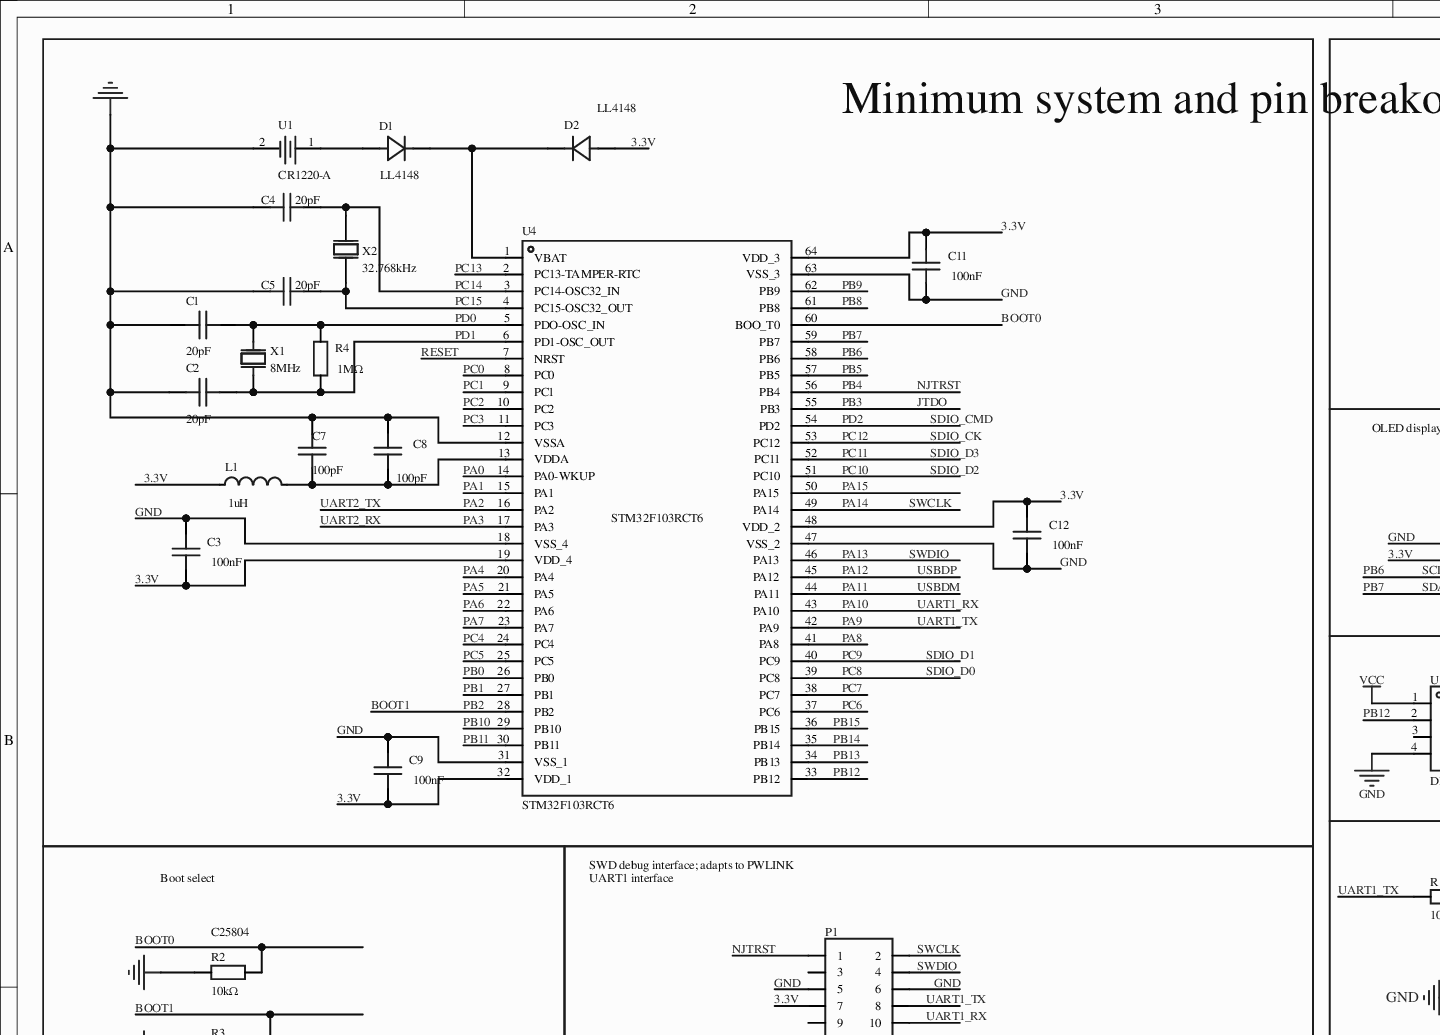
[diagram p0: MISC52064-3.schdoc, top left]
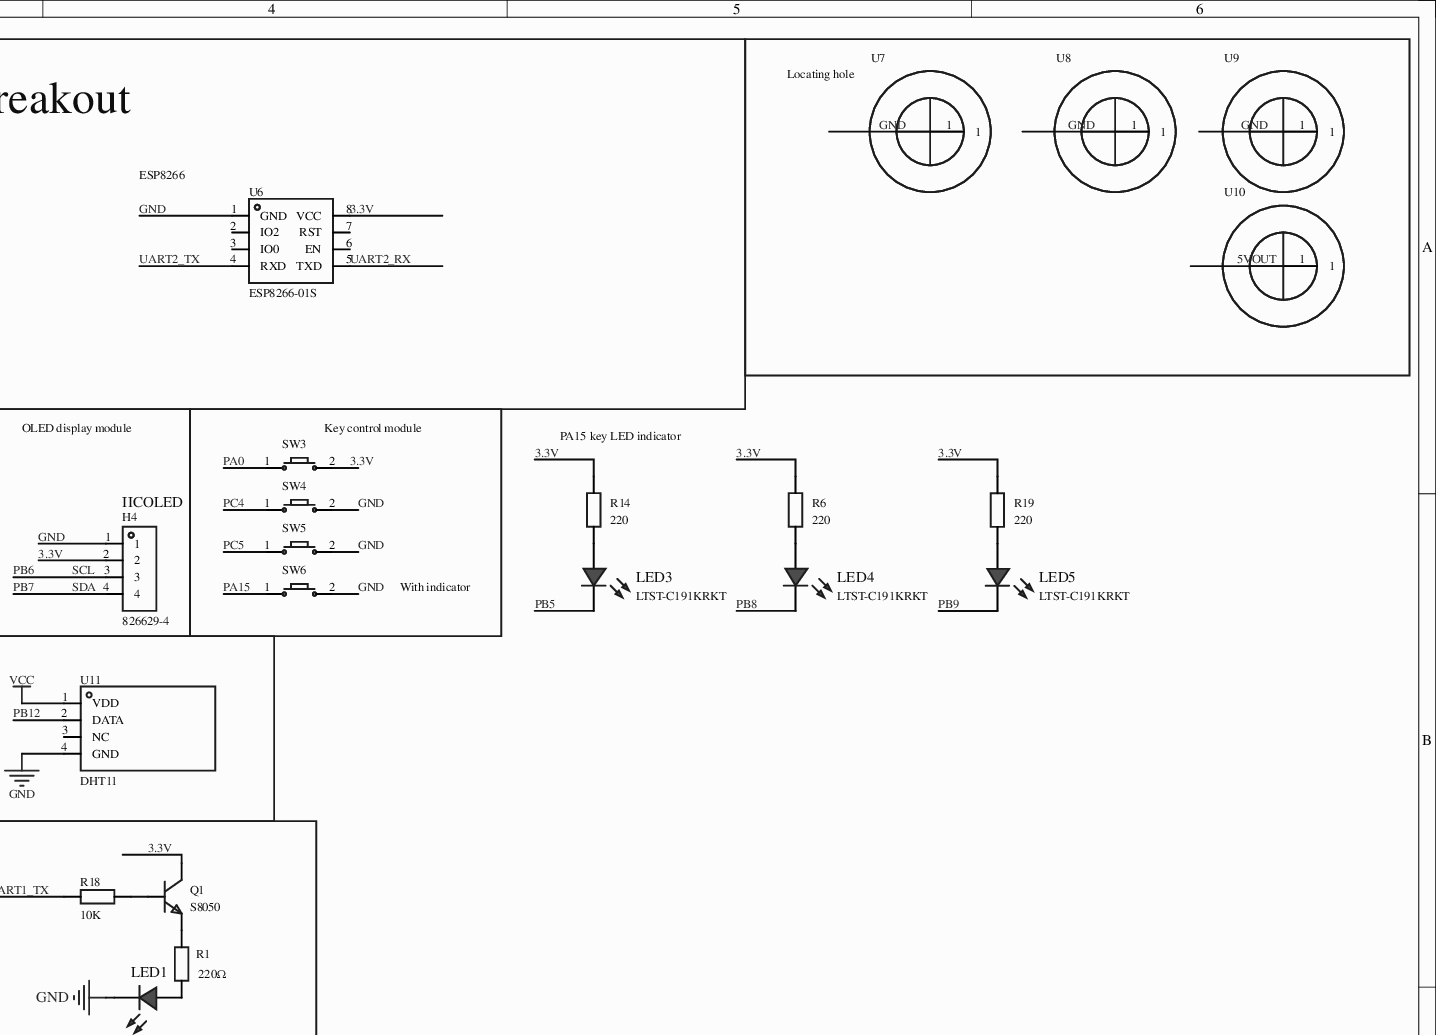
[diagram p1: MISC52064-3.schdoc, top right]
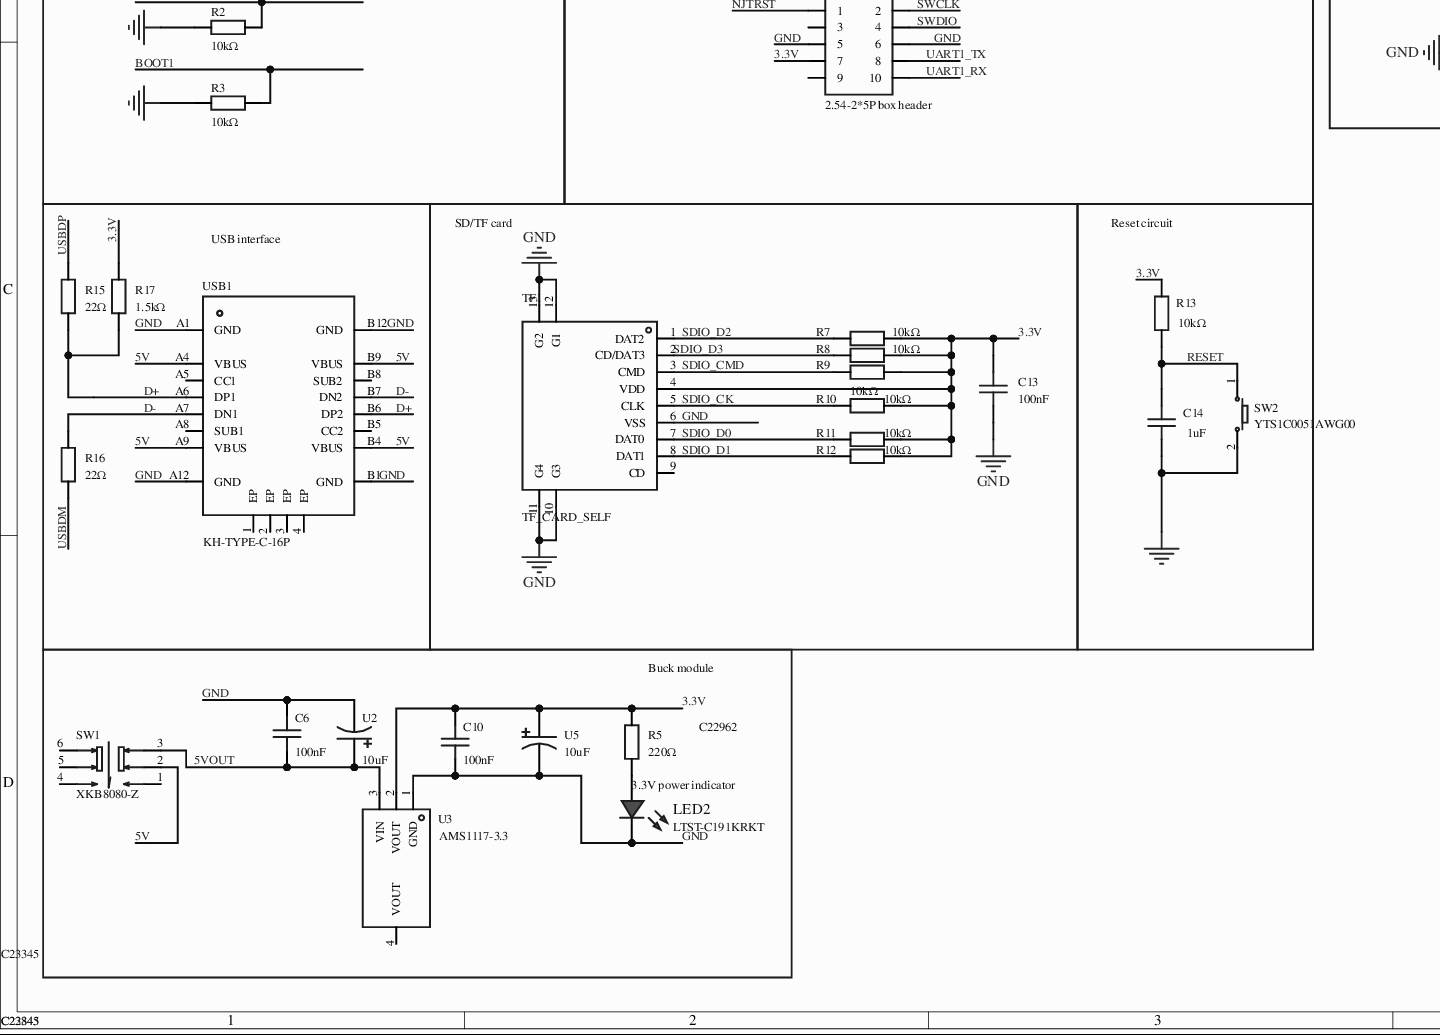
[diagram p2: MISC52064-3.schdoc, bottom left]
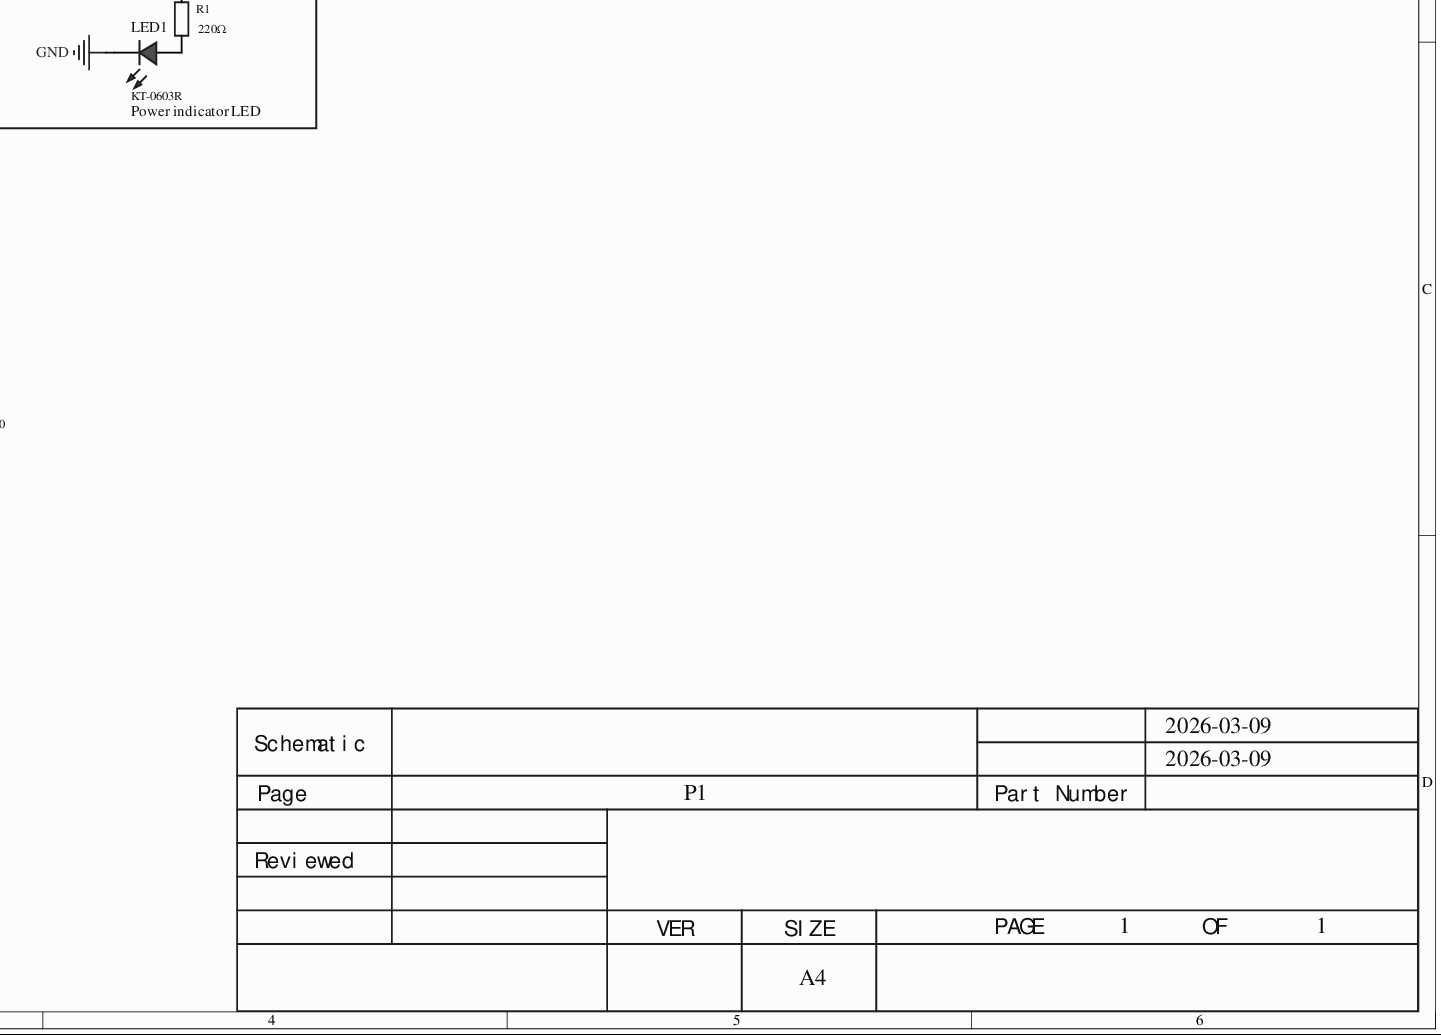
[diagram p3: MISC52064-3.schdoc, bottom right]
# Altium project MISC52064-2.PrjPcb
1 sheet, 65 parts. Net scope: global (net labels, ports and power ports of the same name join across sheets).
Board file: MISC52064.pcbdoc

## Sheet MISC52064-3.schdoc
size 420 x 298 mm; Version: V1.0; @Project Name: MISC52064; @Page Count: 1; @Update Date: 2026-03-09; @Create Date: 2026-03-09; @Schematic Name: MISC52064; @Page No: 1; @Board Name: MISC52064; @Create Time: 16:36:21; @Update Time: 22:44:30

### Parts
C1  20pF  [C0603]
C2  20pF  [C0603]
C3  100nF  [C0603]
C4  20pF  [C0603]
C5  20pF  [C0603]
C6  100nF  [C0603]
C7  100pF  [C0603]
C8  100pF  [C0603]
C9  100nF  [C0603]
C10  100nF  [C0603]
C11  100nF  [C0603]
C12  100nF  [C0603]
C13  100nF  [C0603]
C14  1uF  [C0603]
D1  LL4148  [LL-34_L3.5-W1.5-RD]
D2  LL4148  [LL-34_L3.5-W1.5-RD]
H4  826629-4  用途: IICOLED  [HDR-TH_4P-P2.54-V-M-1]
L1  1uH  [L0603]
LED1  KT-0603R  用途: Power indicator LED  [LED0603-RD]
LED2  LTST-C191KRKT  [LED0603-RD]
LED3  LTST-C191KRKT  [LED0603-RD]
LED4  LTST-C191KRKT  [LED0603-RD]
LED5  LTST-C191KRKT  [LED0603-RD]
P1  2.54-2*5P box header  [IDC-TH_10P-P2.54_C5665]
Q1  S8050  [SOT-23-3_L2.9-W1.3-P1.90-LS2.4-BR]
R1  220Ω  [R0603]
R2  10kΩ  Supplier Part: C25804  [R0603]
R3  10kΩ  [R0603]
R4  1MΩ  [R0603]
R5  220Ω  Supplier Part: C22962  [R0603]
R6  220  [R0603]
R7  10kΩ  [R0603]
R8  10kΩ  [R0603]
R9  10kΩ  [R0603]
R10  10kΩ  [R0603]
R11  10kΩ  [R0603]
R12  10kΩ  [R0603]
R13  10kΩ  [R0603]
R14  220  [R0603]
R15  22Ω  Supplier Part: C23345  [R0603]
R16  22Ω  Supplier Part: C23345  [R0603]
R17  1.5kΩ  Supplier Part: C22843  [R0603]
R18  10K  [R0603]
R19  220  [R0603]
SW1  XKB8080-Z  [SW-TH_6P-L8.0-W8.0-P2.50]
SW2  YTS1C0051AWG00  [SW-SMD_L6.1-W3.6-LS8.0]
SW3  YTS1C0051AWG00  [SW-SMD_L6.1-W3.6-LS8.0]  (value not drawn)
SW4  YTS1C0051AWG00  [SW-SMD_L6.1-W3.6-LS8.0]  (value not drawn)
SW5  YTS1C0051AWG00  [SW-SMD_L6.1-W3.6-LS8.0]  (value not drawn)
SW6  YTS1C0051AWG00  [SW-SMD_L6.1-W3.6-LS8.0]  (value not drawn)
TF1  TF_CARD_SELF  [TF-SMD_TF-15-15]
U1  CR1220-A  [BAT-SMD_CR1220-2]
U2  10uF  [CASE-A_3216]
U3  AMS1117-3.3  [SOT-223-3_L6.5-W3.4-P2.30-LS7.0-BR]
U4  STM32F103RCT6  [LQFP-64_L10.0-W10.0-P0.50-LS12.0-BL]
U5  10uF  [CASE-A_3216]
U6  ESP8266-01S  [WIFIM-TH_ESP8266-01S]
U7  (no value)  [M3_花孔]
U8  (no value)  [M3_花孔]
U9  (no value)  [M3_花孔]
U10  (no value)  [M3_花孔]
U11  DHT11  [SENSOR-TH_DHT11]
USB1  KH-TYPE-C-16P  [USB-C-SMD_KH-TYPE-C-16P]
X1  8MHz  [HC-49S_L11.4-W4.8]
X2  32.768kHz  [OSC-TH_BD2.0-P0.70-D0.3]

### Blocks framed on the sheet
Minimum system and pin breakout: C1-C5 C7-C9 C11 C12 D1 D2 L1 R4 U1 U4 X1 X2
ESP8266: U6
Locating hole: U7-U10
OLED display module: H4
Boot select: R2 R3
USB interface: R15-R17 USB1
SD/TF card: C13 R7-R12 TF1
Reset circuit: C14 R13 SW2

### Nets
GND: C1.1 C2.1 C3.2 C4.1 C5.1 C6.2 C7.2 C8.2 C9.2 C10.1 C11.1 C12.1 C13.1 C14.1 H4.1 LED1.1(C) LED2.1(C) P1.5 P1.6 R2.1 R3.1 SW2.2 SW4.2 SW5.2 SW6.2 TF1.6(VSS) TF1.10(G3) TF1.11(G4) TF1.12(G1) TF1.13(G2) U1.2 U2.2 U3.1(GND) U4.12(VSSA) U4.18(VSS_4) U4.31(VSS_1) U4.47(VSS_2) U4.63(VSS_3) U5.2 U6.1(GND) U7.1 U8.1 U9.1 U11.4(GND) USB1.A1(GND) USB1.A12(GND) USB1.B1(GND) USB1.B12(GND)
VCC: U11.1(VDD)
3.3V: C3.1 C9.1 C10.2 C11.2 C12.2 C13.2 D2.2(A) H4.2 L1.1 P1.7 Q1.3 R5.2 R6.2 R7.2 R8.2 R9.2 R10.2 R11.2 R12.2 R13.2 R14.2 R17.2 R19.2 SW3.2 TF1.4(VDD) U3.2(VOUT) U4.19(VDD_4) U4.32(VDD_1) U4.48(VDD_2) U4.64(VDD_3) U5.1 U6.8(VCC)
5V: SW1.2 USB1.A4(VBUS) USB1.A9(VBUS) USB1.B4(VBUS) USB1.B9(VBUS)
5VOUT: C6.1 SW1.3 U2.1 U3.3(VIN) U10.1
BOOT0: R2.2 U4.60(BOO_T0)
BOOT1: R3.2 U4.28(PB2)  [also labelled PB2]
D+: R15.1 R17.1 USB1.A6(DP1) USB1.B6(DP2)
D-: R16.2 USB1.A7(DN1) USB1.B7(DN2)
JTDO: U4.55(PB3)  [also labelled PB3]
NJTRST: P1.1 U4.56(PB4)  [also labelled PB4]
PA0: SW3.1 U4.14(PA0-WKUP)
PA1: U4.15(PA1)
PA2: U4.16(PA2) U6.4(RXD)  [also labelled UART2_TX]
PA3: U4.17(PA3) U6.5(TXD)  [also labelled UART2_RX]
PA4: U4.20(PA4)
PA5: U4.21(PA5)
PA6: U4.22(PA6)
PA7: U4.23(PA7)
PA8: U4.41(PA8)
PA9: P1.8 R18.1 U4.42(PA9)  [also labelled UART1_TX]
PA10: P1.10 U4.43(PA10)  [also labelled UART1_RX]
PA11: R16.1 U4.44(PA11)  [also labelled USBDM]
PA12: R15.2 U4.45(PA12)  [also labelled USBDP]
PA13: P1.4 U4.46(PA13)  [also labelled SWDIO]
PA14: P1.2 U4.49(PA14)  [also labelled SWCLK]
PA15: SW6.1 U4.50(PA15)
PB0: U4.26(PB0)
PB1: U4.27(PB1)
PB5: LED3.1(C) U4.57(PB5)
PB6: H4.3 U4.58(PB6)  [also labelled SCL]
PB7: H4.4 U4.59(PB7)  [also labelled SDA]
PB8: LED4.1(C) U4.61(PB8)
PB9: LED5.1(C) U4.62(PB9)
PB10: U4.29(PB10)
PB11: U4.30(PB11)
PB12: U4.33(PB12) U11.2(DATA)
PB13: U4.34(PB13)
PB14: U4.35(PB14)
PB15: U4.36(PB15)
PC0: U4.8(PC0)
PC1: U4.9(PC1)
PC2: U4.10(PC2)
PC3: U4.11(PC3)
PC4: SW4.1 U4.24(PC4)
PC5: SW5.1 U4.25(PC5)
PC6: U4.37(PC6)
PC7: U4.38(PC7)
PC8: R11.1 TF1.7(DAT0) U4.39(PC8)  [also labelled SDIO_D0]
PC9: R12.1 TF1.8(DAT1) U4.40(PC9)  [also labelled SDIO_D1]
PC10: R7.1 TF1.1(DAT2) U4.51(PC10)  [also labelled SDIO_D2]
PC11: R8.1 TF1.2(CD/DAT3) U4.52(PC11)  [also labelled SDIO_D3]
PC12: R10.1 TF1.5(CLK) U4.53(PC12)  [also labelled SDIO_CK]
PC13: U4.2(PC13-TAMPER-RTC)
PC14: C4.2 U4.3(PC14-OSC32_IN) X2.1(OSC1)
PC15: C5.2 U4.4(PC15-OSC32_OUT) X2.2(OSC2)
PD0: C1.2 R4.2 U4.5(PDO-OSC_IN) X1.2(OSC2)
PD1: C2.2 R4.1 U4.6(PD1-OSC_OUT) X1.1(OSC1)
PD2: R9.1 TF1.3(CMD) U4.54(PD2)  [also labelled SDIO_CMD]
RESET: C14.2 R13.1 SW2.1 U4.7(NRST)
NetC7_1: C7.1 C8.1 L1.2 U4.13(VDDA)
NetD1_1: D1.1(K) D2.1(K) U4.1(VBAT)
NetD1_2: D1.2(A) U1.1
NetLED1_2: LED1.2(A) R1.1
NetLED2_2: LED2.2(A) R5.1
NetLED3_2: LED3.2(A) R14.1
NetLED4_2: LED4.2(A) R6.1
NetLED5_2: LED5.2(A) R19.1
NetQ1_1: Q1.1 R18.2
NetQ1_2: Q1.2 R1.2

Not connected (* = marked no-connect by the designer): P1 3* 9*; SW1 1* 4* 5* 6*; TF1 9(CD)*; U3 4(VOUT)*; U6 2(IO2) 3(IO0) 6(EN) 7(RST); U11 3(NC); USB1 1(EP)* 2(EP)* 3(EP)* 4(EP)* A5(CC1)* A8(SUB1)* B5(CC2)* B8(SUB2)*

### Notes on the sheet
- (near SW3) Key control module
- (near R14) PA15 key LED indicator
- With indicator
- SWD debug interface; adapts to PWLINK
  UART1 interface
- (near R5) Buck module
- (near LED2) 3.3V power indicator
- 2026-03-09
- Schematic
- Page
- P1
- Part Number
- Reviewed
- VER
- SIZE
- A4
- PAGE
- 1
- OF

### Library data of the parts
C1 C2 C4 C5 = CL10C200JB8NNNC: Capacitance: 20pF; tolerance: ±5%; rated voltage: 50V; dielectric (temperature coefficient): C0G;; Manufacturer: SAMSUNG(三星); AddInBom: yes; ModelId: ac125912035d415993ca9572d50418b1; ModelName: C0603_L1.6-W0.8-H0.8; ModelTransform: 62.992,31.496,0,0,0,0,0,0,0; Symbol: CapAcitance; Device: CL10C200JB8NNNC; LCSC Part Name: 20pF ±5% 50V; Supplier Part: C1648; Manufacturer Part: CL10C200JB8NNNC; JLCPCB Part Class: Basic Part; Datasheet: https://atta.szlcsc.com/upload/public/pdf/source/20160103/1457707686863.pdf; Supplier: LCSC; Tolerance: ±5%; Voltage Rated: 50V; Temperature Coefficient: C0G; Supplier Footprint: 0603; ConvertToPcb: yes; FootprintName: C0603; Value: 20pF
C3 C6 C9-C13 = CC0603KRX7R9BB104: Capacitance: 100nF; tolerance: ±10%; rated voltage: 50V; dielectric (temperature coefficient): X7R;; Manufacturer: YAGEO(国巨); AddInBom: yes; ModelId: ac125912035d415993ca9572d50418b1; ModelName: C0603_L1.6-W0.8-H0.8; ModelTransform: 62.992,31.496,0,0,0,0,0,0,0; Symbol: CapAcitance; Device: CC0603KRX7R9BB104; LCSC Part Name: 100nF ±10% 50V; JLCPCB Part Class: Basic Part; Supplier: LCSC; Tolerance: ±10%; Voltage Rated: 50V; Temperature Coefficient: X7R; Supplier Footprint: 0603; ConvertToPcb: yes; FootprintName: C0603; Value: 100nF
  C3 C6 C9-C12: Supplier Part: C14663; Manufacturer Part: CC0603KRX7R9BB104; Datasheet: https://atta.szlcsc.com/upload/public/pdf/source/20170116/1484561234239.pdf
  C13: Datasheet: https://atta.szlcsc.com/upload/public/pdf/source/20180910/C282072_33301C7F631E79921B82A8DAC6BCC5B3.pdf; SupplierPart: C14663; ManufacturerPart: CC0603KRX7R9BB104
C7 C8 = CL10C101JB8NNNC: Capacitance: 100pF; tolerance: ±5%; rated voltage: 50V; dielectric (temperature coefficient): C0G;; Manufacturer: SAMSUNG(三星); AddInBom: yes; ModelId: ac125912035d415993ca9572d50418b1; ModelName: C0603_L1.6-W0.8-H0.8; ModelTransform: 62.992,31.496,0,0,0,0,0,0,0; Symbol: CapAcitance; Device: CL10C101JB8NNNC; LCSC Part Name: 100pF ±5% 50V; Supplier Part: C14858; Manufacturer Part: CL10C101JB8NNNC; JLCPCB Part Class: Basic Part; Datasheet: https://atta.szlcsc.com/upload/public/pdf/source/20160103/1457707672333.pdf; Supplier: LCSC; Tolerance: ±5%; Voltage Rated: 50V; Temperature Coefficient: C0G; Supplier Footprint: 0603; ConvertToPcb: yes; FootprintName: C0603; Value: 100pF
C14 = CL10A105KB8NNNC: Capacitance: 1uF; tolerance: ±10%; rated voltage: 50V; dielectric (temperature coefficient): X5R;; Manufacturer: SAMSUNG(三星); AddInBom: yes; ModelId: ac125912035d415993ca9572d50418b1; ModelName: C0603_L1.6-W0.8-H0.8; ModelTransform: 62.992,31.496,0,0,0,0,0,0,0; Symbol: CapAcitance; Device: CL10A105KB8NNNC; LCSC Part Name: 1uF ±10% 50V; Supplier Part: C15849; Manufacturer Part: CL10A105KB8NNNC; JLCPCB Part Class: Basic Part; Datasheet: https://atta.szlcsc.com/upload/public/pdf/source/20160103/1457707679084.pdf; Supplier: LCSC; Tolerance: ±10%; Voltage Rated: 50V; Temperature Coefficient: X5R; Supplier Footprint: 0603; ConvertToPcb: yes; FootprintName: C0603; Value: 1uF
D1 D2 = LL4148_C9808: Diode configuration: -; power: 500mW; DC reverse voltage (Vr): 75V; average rectified current (Io): 200mA; forward voltage (Vf): 1V@10mA; reverse current (Ir): 5uA@75V; reverse recovery time (trr): 4ns; operating temperature: +175℃@(Tj);; Manufacturer: ST(先科); Symbol: D_1N4007; AddInBom: yes; ModelId: 4a6f2309ca4c4217857da1816cccdf69; ModelName: LL-34_L3.5-W1.5; ModelTransform: 133.93674,59.031,0,0,0,0,0,0,0; Device: LL4148_C9808; LCSC Part Name: 75V 200mA 4ns; Supplier Part: C9808; Manufacturer Part: LL4148; JLCPCB Part Class: Basic Part; Datasheet: https://atta.szlcsc.com/upload/public/pdf/source/20121108/1457706554347.pdf; Supplier: LCSC; Diode Configuration: -; Power Dissipation: 500mW; Reverse Voltage (Vr): 75V; Average Rectified Current (Io): 200mA; Forward Voltage (Vf@If): 1V@10mA; Reverse Leakage Current: 5uA@75V; Reverse Recovery Time (trr): 4ns; Operating Temperature: +175℃@(Tj); Supplier Footprint: LL-34; ConvertToPcb: yes; FootprintName: LL-34_L3.5-W1.5-RD
H4 = 826629-4: Number of rows: single row; total pin count: 4; pitch: 2.54mm; pin structure: 1x4P; row spacing: -; mounting type: through-hole; round/square pin: -; rated current: 5A; rated voltage: -; mating pin length: 6.7mm; plastic height: 2.8mm; termination pin length: 3.2mm; contact material: brass; operating temperature range: -65℃~+105℃; color: green;; Manufacturer: TE Connectivity(美国泰科); AddInBom: yes; ModelId: f8e5d153169943fabcf3383e1c9553c6; ModelName: HDR-M-2.54_1x4; ModelTransform: 399.999,100,0,0,0,0,0,0,-118.11; LCSC Part Name: 2.54mm 1x4P 直插; JLCPCB Part Class: Extended Part; Current Rating (Max): 5A; Contact Material: Brass; Operating Temperature Range: -65℃~+105℃; Symbol: 826629-4; Device: 826629-4; SupplierPart: C590277; ManufacturerPart: 826629-4; Supplier Footprint: 插件,P=2.54mm; Datasheet: https://atta.szlcsc.com/upload/public/pdf/source/20210923/FCC8CD9A04BA2624CF68C067B4A5B53A.pdf; Supplier: LCSC; ConvertToPcb: yes; FootprintName: HDR-TH_4P-P2.54-V-M-1; Number of Rows: Single row; Number of Pins: 4; Pitch: 2.54mm; Pin Structure: 1x4P; Row Spacing: -; Mounting Type: Through-hole; Circluar Pins/Square Pins: -; Voltage Rating (Max): -; Length of Mating Pin: 6.7mm; Insulation Height: 2.8mm; Length of End Connection Pin: 3.2mm; Color: Green
L1 = DFE18SAN1R0MG0L: Inductance: 1uH; tolerance: ±20%; rated current: 1.7A; saturation current (Isat): 2.1A; DC resistance (DCR): 128mΩ;; Manufacturer: muRata(村田); Symbol: SDFL1608S100KTF; AddInBom: yes; ModelId: 2bc5ec593d464d6ba9807aec0b5673c2; ModelName: L0603_L1.6-W0.8-H0.5_BEAD; ModelTransform: 62.992,31.496,0,180,0,0,0.094,0.629,0; Device: DFE18SAN1R0MG0L; LCSC Part Name: 1uH ±20% 1.7A 128mΩ; Supplier Part: C560043; Manufacturer Part: DFE18SAN1R0MG0L; JLCPCB Part Class: Extended Part; Datasheet: https://atta.szlcsc.com/upload/public/pdf/source/20200527/C560043_FBE7DB36A7B149B0DFA49DBF23B20E2B.pdf; Supplier: LCSC; Tolerance: ±20%; Rated Current: 1.7A; Saturation Current (Isat): 2.1A; DC Resistance (DCR): 128mΩ; Q @ Freq: -; Frequency - Self Resonant: -; Ratings: -; Supplier Footprint: 0603; ConvertToPcb: yes; FootprintName: L0603; Value: 1uH
LED1 = KT-0603R: Emitted color: red; diode configuration: -; dominant wavelength: -; color temperature: -; power: -; mounting: -;; Manufacturer: KENTO; Symbol: LED_R; Convert to PCB: yes; 3D Model: 1f0d29a91be547639d425604e9b96ebb; 3D Model Transform: 63.7794,32.283,0,0,0,0,0,0,0; Add into BOM: yes; Supplier Footprint: 0603; Supplier Part: C2286; JLCPCB Part Class: Basic Part; Device: KT-0603R; LCSC Part Name: 红灯; Manufacturer Part: KT-0603R; Datasheet: https://atta.szlcsc.com/upload/public/pdf/source/20160616/1466072038404.pdf; Supplier: LCSC; Emitted Color: Red; Diode Configuration: -; Lens Color: -; Dominant Wavelength: -; Peak Wavelength: -; Color Temperature: -; Luminous Flux (@25℃): -; Forward Current: -; Forward Voltage (VF): -; Luminous Intensity: -; Power Dissipation: -; Viewing Angle: -; Mounting Sytle: -; Operating Temperature: -40℃~+85℃; FootprintName: LED0603-RD; ModelName: LED0603-RD
LED2 LED3 = LTST-C191KRKT: Emitted color: red; diode configuration: -; dominant wavelength: 631nm; color temperature: -; power: 75mW; mounting: -;; Manufacturer: LITEON(光宝); Symbol: LED_R; Convert to PCB: yes; 3D Model: 1f0d29a91be547639d425604e9b96ebb; 3D Model Transform: 63.7794,32.283,0,0,0,0,0,0,0; Lens Color: Colorless transparent; Peak Wavelength: 639nm; Forward Current: 20mA; Viewing Angle: 130°; Device: LTST-C191KRKT; Add into BOM: yes; Supplier Footprint: 0603; Supplier Part: C125099; JLCPCB Part Class: Extended Part; LCSC Part Name: 红灯; ManufacturerPart: LTST-C191KRKT; Datasheet: https://atta.szlcsc.com/upload/public/pdf/source/20180129/C125099_15171878294931315872.pdf; Supplier: LCSC; FootprintName: LED0603-RD; ModelName: LED0603-RD; Emitted Color: Red; Diode Configuration: -; Dominant Wavelength: 631nm; Color Temperature: -; Power Dissipation: 75mW; Mounting Sytle: -; Operating Temperature: -55℃~+85℃
LED4 LED5 = LTST-C191KRKT: Emitted color: red; diode configuration: -; dominant wavelength: 631nm; color temperature: -; power: 75mW; mounting: -;; Manufacturer: LITEON(光宝); Symbol: LED_R; Lens Color: Colorless transparent; Peak Wavelength: 639nm; Forward Current: 20mA; Viewing Angle: 130°; Convert to PCB: yes; 3D Model: 1f0d29a91be547639d425604e9b96ebb; 3D Model Transform: 63.7794,32.283,0,0,0,0,0,0,0; Device: LTST-C191KRKT; LCSC Part Name: 红灯; Manufacturer Part: LTST-C191KRKT; Datasheet: https://atta.szlcsc.com/upload/public/pdf/source/20180129/C125099_15171878294931315872.pdf; Supplier: LCSC; Emitted Color: Red; Diode Configuration: -; Dominant Wavelength: 631nm; Color Temperature: -; Power Dissipation: 75mW; Mounting Sytle: -; Operating Temperature: -55℃~+85℃; Add into BOM: yes; Supplier Footprint: 0603; Supplier Part: C125099; JLCPCB Part Class: Extended Part; FootprintName: LED0603-RD; ModelName: LED0603-RD
P1 = 2.54-2*5P简牛: Connector type: box header; pins per row: 5; rows: 2; pitch: 2.54mm; row spacing: 2.54mm; package: through-hole; contact material: -; contact plating: -;; Manufacturer: BOOMELE(博穆精密); Symbol: HDR-IDC-2.54-2X5P; AddInBom: yes; ModelId: 1d28e50a904749439e5167098e48e984; ModelTransform: 799.998,348.41478,0,0,0,0,0,3.937,-118.11; Pin Number in each Row: 5; Device: 2.54-2*5P box header; LCSC Part Name: 每排P数:5 排数:2 2.54mm; SupplierPart: C5665; ManufacturerPart: 2.54-2*5P简牛; Supplier Footprint: 插件,P=2.54mm; JLCPCB Part Class: Extended Part; Datasheet: https://atta.szlcsc.com/upload/public/pdf/source/20140331/1457707037896.pdf; Supplier: LCSC; ConvertToPcb: yes; FootprintName: IDC-TH_10P-P2.54_C5665; ModelName: HDR-IDC-2.54-2X5P; Connector Type: Box header; Number of Rows: 2; Pitch: 2.54mm; Row Spacing: 2.54mm; Holder Type: Through-hole; Contact Material: -; Contact Plating: -
Q1 = S8050_C2762211: Transistor type: NPN; collector-emitter breakdown voltage (Vceo): 25V; collector current (Ic): 500mA; power (Pd): 300mW; collector-emitter saturation voltage (VCE(sat)@Ic,Ib): 600mV@500mA,50mA; DC current gain (hFE@Ic,Vce): 120@50mA,1V; transition frequency (fT): 150MHz; operating temperature: -55℃~+150℃@(Tj);; Manufacturer: 晶导微电子; AddInBom: yes; ModelId: c62791f0466c4ae2a892c056b845b0ca; ModelName: SOT-23-3P_L2.9-W1.3-H1.0-LS2.4-P0.95; ModelTransform: 98.425,114.173,0,180,0,0,0.0005,-0.0005,0; Symbol: NPN; Device: S8050_C2762211; LCSC Part Name: S8050; SupplierPart: C2762211; ManufacturerPart: S8050; Supplier Footprint: SOT-23; JLCPCB Part Class: Extended Part; Datasheet: https://atta.szlcsc.com/upload/public/pdf/source/20210521/C2762211_5AC5D762C14CC7F013712CBEE509B0DC.pdf; Supplier: LCSC; ConvertToPcb: yes; FootprintName: SOT-23-3_L2.9-W1.3-P1.90-LS2.4-BR; Transistor Type: NPN; Collector-Emitter Breakdown Voltage (Vceo): 25V; Collector Current (Ic): 500mA; Power Dissipation (Pd): 300mW; Collector-Emitter Saturation Voltage (VCE(sat)@Ic,Ib): 600mV@500mA,50mA; DC Current Gain (hFE@Ic,Vce): 120@50mA,1V; Transition Frequency (fT): 150MHz; Operating Temperature: -55℃~+150℃@(Tj)
R1 = 0603WAF2200T5E: Resistor type: thick film resistor; resistance: 220Ω; tolerance: ±1%; power: 100mW; temperature coefficient: ±100ppm/℃; max working voltage: 75V; operating temperature range: -55℃~+155℃;; Manufacturer: UNI-ROYAL(厚声); AddInBom: yes; ModelId: 6bd5cd867e9542ebae21caaf5d2d4c4d; ModelTransform: 31.8897,63.7794,0,90,0,0,0,0,0; Symbol: Resistor; Device: 0603WAF2200T5E; LCSC Part Name: 220Ω ±1% 100mW; Supplier Part: C22962; Manufacturer Part: 0603WAF2200T5E; JLCPCB Part Class: Basic Part; Datasheet: https://atta.szlcsc.com/upload/public/pdf/source/20200306/C422600_1E6D84923E4A46A82E41ADD87F860B5C.pdf; Supplier: LCSC; Type: Thick film resistor; Tolerance: ±1%; Power(Watts): 100mW; Temperature Coefficient: ±100ppm/℃; Overload Voltage (Max): 75V; Operating Temperature Range: -55℃~+155℃; Supplier Footprint: 0603; ConvertToPcb: yes; FootprintName: R0603; ModelName: R0603; Value: 220Ω
R2 R7-R12 R14 = 0603WAF1002T5E: Resistor type: thick film resistor; resistance: 10kΩ; tolerance: ±1%; power: 100mW;; Manufacturer: UNI-ROYAL(厚声); 3D Model: fc143cca1e79419f9cd78b61e9279f08; AddInBom: yes; ModelTransform: 31.8897,63.7794,0,90,0,0,0,0,0; Temperature Coefficient: ±100ppm/℃; Overload Voltage (Max): 75V; Symbol: Resistor; Device: 0603WAF1002T5E; LCSC Part Name: 厚膜电阻 10kΩ ±1% 100mW; JLCPCB Part Class: Basic Part; ManufacturerPart: 0603WAF1002T5E; Supplier Footprint: 0603; Datasheet: https://atta.szlcsc.com/upload/public/pdf/source/20200306/C422600_1E6D84923E4A46A82E41ADD87F860B5C.pdf; Supplier: LCSC; ConvertToPcb: yes; FootprintName: R0603; ModelName: R0603; Type: Thick film resistor; Tolerance: ±1%; Power(Watts): 100mW; Operating Temperature Range: -55℃~+155℃
  R2: Value: 10kΩ
  R7-R12: SupplierPart: C25804; Value: 10kΩ
  R14: Value: 220
R3 = 0603WAF1002T5E: Resistor type: thick film resistor; resistance: 10kΩ; tolerance: ±1%; power: 100mW;; Manufacturer: UNI-ROYAL(厚声); 3D Model: fc143cca1e79419f9cd78b61e9279f08; Temperature Coefficient: ±100ppm/℃; AddInBom: yes; ModelTransform: 31.8897,63.7794,0,90,0,0,0,0,0; Overload Voltage (Max): 75V; Symbol: Resistor; Device: 0603WAF1002T5E; LCSC Part Name: 厚膜电阻 10kΩ ±1% 100mW; Supplier Part: C25804; Manufacturer Part: 0603WAF1002T5E; JLCPCB Part Class: Basic Part; Datasheet: https://atta.szlcsc.com/upload/public/pdf/source/20200306/C422600_1E6D84923E4A46A82E41ADD87F860B5C.pdf; Supplier: LCSC; Power(Watts): 100mW; Tolerance: ±1%; Operating Temperature Range: -55℃~+155℃; Supplier Footprint: 0603; ConvertToPcb: yes; FootprintName: R0603; ModelName: R0603; Type: Thick film resistor; Value: 10kΩ
R4 = 0603WAF1004T5E: Resistor type: thick film resistor; resistance: 1MΩ; tolerance: ±1%; power: 100mW;; Manufacturer: UNI-ROYAL(厚声); 3D Model: fc143cca1e79419f9cd78b61e9279f08; Temperature Coefficient: ±100ppm/℃; Overload Voltage (Max): 75V; AddInBom: yes; ModelTransform: 31.8897,63.7794,0,90,0,0,0,0,0; Symbol: Resistor; Value: 1MΩ; Device: 0603WAF1004T5E; LCSC Part Name: 1MΩ ±1% 100mW; Supplier Part: C22935; Manufacturer Part: 0603WAF1004T5E; JLCPCB Part Class: Basic Part; Datasheet: https://atta.szlcsc.com/upload/public/pdf/source/20200306/C422600_1E6D84923E4A46A82E41ADD87F860B5C.pdf; Supplier: LCSC; Type: Thick film resistor; Tolerance: ±1%; Power(Watts): 100mW; Operating Temperature Range: -55℃~+155℃; Supplier Footprint: 0603; ConvertToPcb: yes; FootprintName: R0603; ModelName: R0603
R5 = 0603WAF2200T5E: Resistor type: thick film resistor; resistance: 220Ω; tolerance: ±1%; power: 100mW;; Manufacturer: UNI-ROYAL(厚声); 3D Model: fc143cca1e79419f9cd78b61e9279f08; AddInBom: yes; ModelTransform: 31.8897,63.7794,0,90,0,0,0,0,0; Temperature Coefficient: ±100ppm/℃; Overload Voltage (Max): 75V; Symbol: Resistor; Device: 0603WAF2200T5E; LCSC Part Name: 220Ω ±1% 100mW; JLCPCB Part Class: Basic Part; ManufacturerPart: 0603WAF2200T5E; Supplier Footprint: 0603; Datasheet: https://atta.szlcsc.com/upload/public/pdf/source/20200306/C422600_1E6D84923E4A46A82E41ADD87F860B5C.pdf; Supplier: LCSC; ConvertToPcb: yes; FootprintName: R0603; ModelName: R0603; Type: Thick film resistor; Value: 220Ω; Tolerance: ±1%; Power(Watts): 100mW; Operating Temperature Range: -55℃~+155℃
R6 R19 = 0603WAF1002T5E: Resistor type: thick film resistor; resistance: 10kΩ; tolerance: ±1%; power: 100mW;; Manufacturer: UNI-ROYAL(厚声); 3D Model: fc143cca1e79419f9cd78b61e9279f08; 3D Model Transform: 31.8897,63.7794,0,90,0,0,0,0,0; Temperature Coefficient: ±100ppm/℃; Overload Voltage (Max): 75V; AddInBom: yes; Symbol: Resistor; Device: 0603WAF1002T5E; LCSC Part Name: 厚膜电阻 10kΩ ±1% 100mW; JLCPCB Part Class: Basic Part; Manufacturer Part: 0603WAF1002T5E; Supplier Footprint: 0603; Datasheet: https://atta.szlcsc.com/upload/public/pdf/source/20200306/C422600_1E6D84923E4A46A82E41ADD87F860B5C.pdf; Supplier: LCSC; Type: Thick film resistor; Value: 220; Tolerance: ±1%; Power(Watts): 100mW; Operating Temperature Range: -55℃~+155℃; ConvertToPcb: yes; FootprintName: R0603; ModelName: R0603
R13 = 0603WAF1002T5E: Resistor type: thick film resistor; resistance: 10kΩ; tolerance: ±1%; power: 100mW; temperature coefficient: ±100ppm/℃; max working voltage: 75V; operating temperature range: -55℃~+155℃;; Manufacturer: UNI-ROYAL(厚声); AddInBom: yes; ModelId: 6bd5cd867e9542ebae21caaf5d2d4c4d; ModelTransform: 31.8897,63.7794,0,90,0,0,0,0,0; Symbol: Resistor; Device: 0603WAF1002T5E; LCSC Part Name: 10kΩ ±1% 100mW; Supplier Part: C25804; Manufacturer Part: 0603WAF1002T5E; JLCPCB Part Class: Basic Part; Datasheet: https://atta.szlcsc.com/upload/public/pdf/source/20200306/C422600_1E6D84923E4A46A82E41ADD87F860B5C.pdf; Supplier: LCSC; Type: Thick film resistor; Tolerance: ±1%; Power(Watts): 100mW; Temperature Coefficient: ±100ppm/℃; Overload Voltage (Max): 75V; Operating Temperature Range: -55℃~+155℃; Supplier Footprint: 0603; ConvertToPcb: yes; FootprintName: R0603; ModelName: R0603; Value: 10kΩ
R15 R16 = 0603WAF220JT5E: Resistor type: thick film resistor; resistance: 22Ω; tolerance: ±1%; power: 100mW;; Manufacturer: UNI-ROYAL(厚声); AddInBom: yes; ModelId: fc143cca1e79419f9cd78b61e9279f08; ModelTransform: 31.8897,63.7794,0,90,0,0,0,0,0; Temperature Coefficient: ±100ppm/℃; Overload Voltage (Max): 75V; Symbol: Resistor; Device: 0603WAF220JT5E; LCSC Part Name: 22Ω ±1% 100mW; ManufacturerPart: 0603WAF220JT5E; Supplier Footprint: 0603; JLCPCB Part Class: Basic Part; Datasheet: https://atta.szlcsc.com/upload/public/pdf/source/20200306/C422600_1E6D84923E4A46A82E41ADD87F860B5C.pdf; Supplier: LCSC; ConvertToPcb: yes; FootprintName: R0603; ModelName: R0603; Type: Thick film resistor; Value: 22Ω; Tolerance: ±1%; Power(Watts): 100mW; Operating Temperature Range: -55℃~+155℃
R17 = 0603WAF1501T5E: Resistor type: thick film resistor; resistance: 1.5kΩ; tolerance: ±1%; power: 100mW;; Manufacturer: UNI-ROYAL(厚声); AddInBom: yes; ModelId: fc143cca1e79419f9cd78b61e9279f08; ModelTransform: 31.8897,63.7794,0,90,0,0,0,0,0; Temperature Coefficient: ±100ppm/℃; Overload Voltage (Max): 75V; Symbol: Resistor; Device: 0603WAF1501T5E; LCSC Part Name: 1.5kΩ ±1% 100mW; ManufacturerPart: 0603WAF1501T5E; Supplier Footprint: 0603; JLCPCB Part Class: Basic Part; Datasheet: https://atta.szlcsc.com/upload/public/pdf/source/20200306/C422600_1E6D84923E4A46A82E41ADD87F860B5C.pdf; Supplier: LCSC; ConvertToPcb: yes; FootprintName: R0603; ModelName: R0603; Type: Thick film resistor; Value: 1.5kΩ; Tolerance: ±1%; Power(Watts): 100mW; Operating Temperature Range: -55℃~+155℃
R18 = Res_0603: Symbol: Resistor; ConvertToPcb: yes; ModelId: 6bd5cd867e9542ebae21caaf5d2d4c4d; ModelTransform: 31.8897,63.7794,0,90,0,0,0,0,0; Device: Res_0603; AddInBom: yes; Supplier Footprint: 0603; FootprintName: R0603; ModelName: R0603; Value: 10K
SW1 = XKB8080-Z: Contact current: 100mA; rated voltage (AC): 250V; rated voltage (DC): 30V; insulation resistance: 100MΩ; mounting: through-hole; self-lock/no-lock: self-lock; actuator shape: rectangular button; actuator/cap color: blue; lamp: none; pin style: PC pin; actuating force: 160gf@±80gf; protection rating: -; operating temperature: -15℃~+55℃; mechanical life: 100000;; Manufacturer: XKB Connectivity(中国星坤); Symbol: XKB7070-Z; 3D Model: 82e4a315926f45d0a816f91690893dc00819f05c4eef4c71ace90d822a990e87; 3D Model Transform: 275.59,275.629,0,0,0,0,0,0,-137.795; AddInBom: yes; ModelName: SW-TH_6P-L7.0-W7.0-P2.00; Pin Style: PC pin; Mechanical Life: 100000; Device: XKB8080-Z; Circuit: -; LCSC Part Name: 8*8 蓝白黑 自锁开关; SupplierPart: C318860; ManufacturerPart: XKB8080-Z; Supplier Footprint: 插件; JLCPCB Part Class: Extended Part; Datasheet: https://atta.szlcsc.com/upload/public/pdf/source/20200227/C318860_5054FF4F05FC2BEF6D52FB06C07EBD2C.pdf; Supplier: LCSC; ConvertToPcb: yes; FootprintName: SW-TH_6P-L8.0-W8.0-P2.50; Contact Current: 100mA; Voltage Rating (AC): 250V; Voltage Rating (DC): 30V; Insulation Resistance: 100MΩ; Mounting Style: Through-hole; Self Lock / No Lock: Self-lock; Actuator Style: Rectangular button; Actuator/Cap Color: Blue; With Lamp: None; Operating Force: 160gf@±80gf; IP Rating: -; Operating Temperature: -15℃~+55℃
SW2-SW6 = YTS1C0051AWG00: Switch length: 6.1mm; switch width: 3.6mm; switch height: 2.5mm;; Manufacturer: YIYUAN(怡远); Symbol: Tactile switch x2; AddInBom: yes; ModelId: aaf790cb4e294df09db9105c4bdc187b; ModelName: KEY-SMD_2P-L6.1-W3.7-H2.5-LS8.0; ModelTransform: 311.023,141.732,0,0,0,0,0,0,0; Device: YTS1C0051AWG00; LCSC Part Name: 白色按键头3.6x6.1x2.5 180gf两脚贴片; SupplierPart: C5159017; ManufacturerPart: YTS1C0051AWG00; Supplier Footprint: SMD; JLCPCB Part Class: Extended Part; Datasheet: https://atta.szlcsc.com/upload/public/pdf/source/20220909/90D1F3506E0247DF6BB595157A95988A.pdf; Supplier: LCSC; ConvertToPcb: yes; FootprintName: SW-SMD_L6.1-W3.6-LS8.0; Switch Length: 6.1mm; Switch Width: 3.6mm; Switch Height: 2.5mm
TF1 = TF_CARD_SELF: AddInBom: yes; ModelId: 67496f576e2f431c95a797a452f0eadc; ModelTransform: 598.424,635.826,0,0,0,0,79.804,8.934,-23.622; Device: TF_CARD_SELF; Symbol: TF_CARD_SELF; LCSC Part Name: TF_CARD_SELF; SupplierPart: C9900010414; ManufacturerPart: TF_CARD_SELF; Supplier Footprint: TFCARD; JLCPCB Part Class: Extended library; Supplier: LCSC; ConvertToPcb: yes; FootprintName: TF-SMD_TF-15-15; ModelName: TF-SMD_TF-15-15
U1 = CR1220-A: AddInBom: yes; ModelId: aa69efc108b9406287881e5b236f6e7a; ModelTransform: 777.81069,586.46209,0,180,0,0,-19.685,0,-31.496; Device: CR1220-A; Symbol: CR1220-A; LCSC Part Name: CR1220-A; SupplierPart: C9900016718; ManufacturerPart: CR1220-A; Supplier Footprint: SMD-2P; JLCPCB Part Class: Extended library; Supplier: LCSC; ConvertToPcb: yes; FootprintName: BAT-SMD_CR1220-2; ModelName: BAT-SMD_CR1220-2
U2 U5 = NOJA106M006RWJ: Capacitance: 10uF; tolerance: ±20%; rated voltage: 6.3V; leakage current: 1.2uA; ESR: 2.2Ω@100kHz; dissipation factor: 6%; operating temperature: -55℃~+105℃;; Manufacturer: Kyocera AVX; AddInBom: yes; ModelId: d42b6f9952ad429a883ac5dd55ff7452; ModelName: CASE-A_L3.2-W1.6-H1.6; ModelTransform: 125.984,62.992,0,0,0,0,-0.003,0,0; Device: NOJA106M006RWJ; Symbol: NOJA106M006RWJ; LCSC Part Name: 10uF ±20% 6.3V; SupplierPart: C145084; ManufacturerPart: NOJA106M006RWJ; Supplier Footprint: CASE-A-3216-18(mm); JLCPCB Part Class: Extended Part; Datasheet: https://atta.szlcsc.com/upload/public/pdf/source/20180125/C145084_15168615115041301546.pdf; Supplier: LCSC; ConvertToPcb: yes; FootprintName: CASE-A_3216; Value: 10uF; Tolerance: ±20%; Rated Voltage: 6.3V; Leakage Current(DCL): 1.2uA; Equivalent Series   Resistance(ESR): 2.2Ω@100kHz; Dissipation Factor: 6%; Operating Temperature: -55℃~+105℃
U3 = AMS1117-3.3_C6186: Output type: fixed; output polarity: positive; output channels: 1; max input voltage: -; output voltage: 3.3V; dropout: 1.3V@(800mA); quiescent current (ground current): -; output current: 1A; power supply ripple rejection (PSRR): 72dB@(120Hz); noise: -; features: -; operating temperature: -;; Manufacturer: AMS; AddInBom: yes; ModelId: 925194bf9823436183a3e0b978a8d076; ModelName: SOT-223-4P_L6.5-W3.5-H1.6-LS7.0-P2.30; ModelTransform: 279.89794,255.905,0,180,0,0,-3.9385,-0.0005,0; Number of Outputs: 1; Device: AMS1117-3.3_C6186; Symbol: AMS1117-3.3; LCSC Part Name: 正Vout=3.3V1A72dB@(120Hz); SupplierPart: C6186; ManufacturerPart: AMS1117-3.3; Supplier Footprint: SOT-223-3; JLCPCB Part Class: Basic library; Datasheet: https://atta.szlcsc.com/upload/public/pdf/source/20180727/C6186_7A095716F0823C02F1997A905E26C086.pdf; Supplier: LCSC; ConvertToPcb: yes; FootprintName: SOT-223-3_L6.5-W3.4-P2.30-LS7.0-BR; Output Type: Fixed; Output Polarity: Positive; Maximum Input Voltage: -; Output Voltage: 3.3V; Dropout Voltage: 1.3V@(800mA); Quiescent Current (Ground Current): -; Output Current: 1A; Power Supply Rejection Ratio (PSRR): 72dB@(120Hz); Noise: -; Feature: -; Operating Temperature: -
U4 = STM32F103RCT6: CPU core: ARM Cortex-M3; CPU max frequency: 72MHz; operating voltage: 2V~3.6V; program memory: 256KB; total RAM: 48KB; EEPROM/data FLASH capacity: 256KB; GPIO count: 51; ADC (bits): 12bit; DAC (bits): 12bit; (E)PWM (bits): -; peripherals/functions: DMA; watchdog; on-chip temperature sensor; PWM; internal oscillator: yes; operating temperature range: -40℃~+85℃;; Manufacturer: ST(意法半导体); ModelId: cd9de06618c44fcf82654c43a457f83c; ModelName: LQFP-64_L10.0-W10.0-H1.4-LS12.0-P0.50; ModelTransform: 472.441,472.441,0,0,0,0,0,0,0; GPIO Ports Number: 51; Symbol: STM32F103RCT6; Device: STM32F103RCT6; LCSC Part Name: ARMCortex-M372MHz; SupplierPart: C8323; ManufacturerPart: STM32F103RCT6; Supplier Footprint: LQFP-64(10x10); JLCPCB Part Class: Extended library; Datasheet: https://atta.szlcsc.com/upload/public/pdf/source/20161130/1480498797345.pdf; Supplier: LCSC; AddInBom: yes; ConvertToPcb: yes; FootprintName: LQFP-64_L10.0-W10.0-P0.50-LS12.0-BL; CPU Core: ARMCortex-M3; CPU Maximum Speed: 72MHz; Operating Voltage Range: 2V~3.6V; Program Storage Size: 256KB; Program Memory Type: FLASH; RAM Size: 48KB; EEPROM: 256KB; ADC (Bit): 12bit; DAC (Bit): 12bit; PWM (Bit): -; Universal Serial Bus: -; Internal Comparator: -; Peripheral/Function: DMA; watchdog; on-chip temperature sensor; PWM; communication protocol: -; Watchdog: -; Real-Time Clock: -; Infrared Data Association: -; Low-Voltage Detect: -; CCP Capture/Compare: -; Secure Digital Input and Output: -; Direct Memory Access: -; Internal Oscillator: Yes; Operating Temperature Range: -40℃~+85℃
U6 = ESP8266-01S: AddInBom: yes; ModelId: 7671a3a19d0d4245ae5d5806b59f4d510819f05c4eef4c71ace90d822a990e87; ModelTransform: 566.928,972.439,0,0,0,0,0,378.464,-118.11; Symbol: ESP8266-01S; Device: ESP8266-01S; LCSC Part Name: ESP8266-01S; SupplierPart: C9900150497; ManufacturerPart: ESP8266-01S; Supplier Footprint: TH-8P; JLCPCB Part Class: Extended Part; Supplier: LCSC; ConvertToPcb: yes; FootprintName: WIFIM-TH_ESP8266-01S; ModelName: WIFIM-TH_ESP8266-01S
U7-U10 = M3孔_花孔: Device: M3 flower hole; Check: false; ConvertToPcb: yes; SymbolName: M3 flower hole; FootprintName: M3_flower hole; AddInBom: yes
U11 = DHT11: Operating temperature range: -20℃~+60℃; humidity range: 5%RH~95%RH; humidity accuracy: ±5%RH;; Manufacturer: 广州奥松; AddInBom: yes; ModelId: 6dde47d4d8bf4fa598dffcc067449c1d0819f05c4eef4c71ace90d822a990e87; ModelTransform: 236.25937,492.125,0,270,0,0,0,-11.811,-196.85; Voltage - Supply: 3.3V~5.5V; Current - Supply: 1mA; Temperature Tolerance: ±2℃; Symbol: DHT11; Device: DHT11; LCSC Part Name: 新款电容式数字温湿度传感器,老款已停产16.1x12.6x5.8mm DHT11  电容式传感器; SupplierPart: C117051; ManufacturerPart: DHT11; Supplier Footprint: SIP-4; JLCPCB Part Class: Extended Part; Datasheet: https://item.szlcsc.com/datasheet/DHT11/118309.html; Supplier: LCSC; ConvertToPcb: yes; FootprintName: SENSOR-TH_DHT11; ModelName: SENSOR-TH_DHT11; Temperature Range: -20℃~+60℃; Humidity: 5%RH~95%RH; Humidity Tolerance: ±5%RH
USB1 = KH-TYPE-C-16P: Connector type: Type-C; standard: -; gender: female; contacts: 16; ports: 1; mounting: flat SMT; rated current - power: 3A; operating temperature range: -40℃~+85℃;; Manufacturer: kinghelm(金航标); Symbol: USB_TYPE-C-16P; Number of Contacts: 16; Number of Ports: 1; AddInBom: yes; ModelId: f2c381012fbf47e0b76dea5162270f01; ModelTransform: 351.9678,307.48,0,0,0,0,0,-45.275,-43.307; Device: KH-TYPE-C-16P; LCSC Part Name: Type-C 母座 卧贴; Supplier Part: C709357; Manufacturer Part: KH-TYPE-C-16P; JLCPCB Part Class: Extended Part; Datasheet: https://atta.szlcsc.com/upload/public/pdf/source/20200911/C709357_AA8DCEB38BB20E3035A7ED7AE7667837.pdf; Supplier: LCSC; Connector Type: Type-C; Standard: -; Gender: Female; Mounting Style: Flat SMT; Current Rating - Power (Max): 3A; Operating Temperature Range: -40℃~+85℃; Supplier Footprint: SMD; ConvertToPcb: yes; FootprintName: USB-C-SMD_KH-TYPE-C-16P; ModelName: USB-C-SMD_KH-TYPE-C-16P
X1 = X49SM8MSB2SC: Crystal type: 49SMD; frequency: 8MHz; frequency tolerance: ±10ppm; frequency stability: ±30ppm; load capacitance: 20pF; operating temperature: -20℃~+70℃;; Manufacturer: YXC(扬兴晶振); AddInBom: yes; ModelId: 6f569b91267b44029b8615eb5c810fba; ModelName: HC-49S_L11.4-W1.8-H3.0-LS12.7; ModelTransform: 499.999,188.976,0,0,0,0,0,0,0; Device: X49SM8MSB2SC; Symbol: X49SM8MSB2SC; LCSC Part Name: HC-49SMD8MHz±10ppm20pF; SupplierPart: C108703; ManufacturerPart: X49SM8MSB2SC; Supplier Footprint: HC-49S-SMD-2P; JLCPCB Part Class: Extended library; Datasheet: https://atta.szlcsc.com/upload/public/pdf/source/20210329/C106809_0E91E60850A780B284B63D653DC40EA4.pdf; Supplier: LCSC; ConvertToPcb: yes; FootprintName: HC-49S_L11.4-W4.8; Crystal Type: 49SMD; Value: 8MHz; Frequency Tolerance: ±10ppm; Frequency Stability: ±30ppm; Load Capacitance: 20pF; Operating Temperature: -20℃~+70℃
X2 = 7S032768NW2: Frequency: 32.768kHz; frequency tolerance: ±20ppm; load capacitance: 12.5pF;; Manufacturer: HD(浩都频率); Symbol: FC-135 32.7680KA-AC; Equivalent Series Resistance (ESR): 70kΩ; AddInBom: yes; ModelId: 7f504e993f4c44b39a6c4ce789f5cee5; ModelName: OSC-TH_D2.0-W6.0-P0.70; ModelTransform: 300.09783,78.682,0,0,0,0,-145.669,-0.005,-137.795; Crystal Type: Cylindrical crystal; Device: 7S032768NW2; LCSC Part Name: 32.768kHz ±20ppm 12.5pF; SupplierPart: C655212; ManufacturerPart: 7S032768NW2; Supplier Footprint: DT-26; JLCPCB Part Class: Extended Part; Datasheet: https://atta.szlcsc.com/upload/public/pdf/source/20220223/405F6AA8E4C09000543E3DD5BF41A4B1.pdf; Supplier: LCSC; ConvertToPcb: yes; FootprintName: OSC-TH_BD2.0-P0.70-D0.3; Value: 32.768kHz; Frequency Tolerance: ±20ppm; Frequency Stability: ±20ppm; Load Capacitance: 12.5pF; Operating Temperature: -